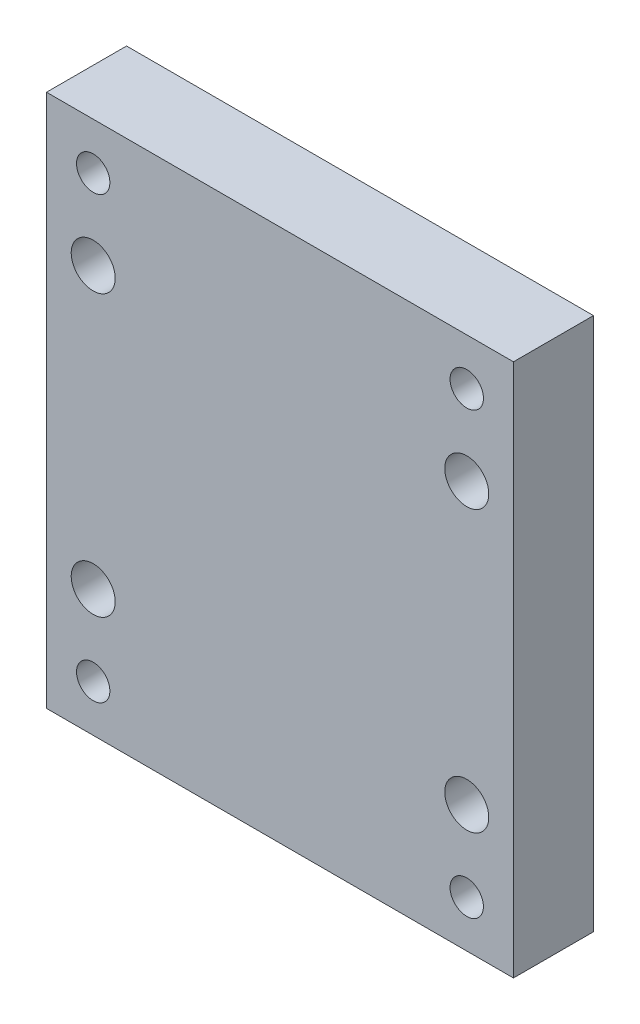
from build123d import *

# Parameters (mm, degrees)
SKETCH_1_W                     = 70
SKETCH_1_H                     = 80
EXTRUDE_1_DEPTH                = 12
HOLE_WIZARD_M6_1_D             = 5
HOLE_WIZARD_M6_1_2_D           = 6.6
HOLE_WIZARD_M6_1_2_CBORE_D     = 11
HOLE_WIZARD_M6_1_2_CBORE_DEPTH = 6.4
CUT_EXTRUDE_1_DEPTH            = 2.5
PATTERN_LINEAR_1_COUNT         = 8
PATTERN_LINEAR_1_PITCH         = 10


with BuildPart() as part:
    # 草图1 → 凸台-拉伸1 (new body)
    with BuildSketch(Plane.XY):
        Rectangle(SKETCH_1_W, SKETCH_1_H)
    extrude(amount=EXTRUDE_1_DEPTH)

    # Hole Wizard M6 _1 (through all)
    with Locations(Plane(origin=(0, 0, 0), x_dir=(-1, 0, 0), z_dir=(0, 0, -1))):
        with Locations((-28, -33), (-28, 33), (28, 33), (28, -33)):
            Hole(HOLE_WIZARD_M6_1_D / 2)

    # Hole Wizard M6 _1 2 (through all)
    with Locations(Plane(origin=(0, 0, 0), x_dir=(-1, 0, 0), z_dir=(0, 0, -1))):
        with Locations((-28, -21), (-28, 21), (28, -21), (28, 21)):
            CounterBoreHole(HOLE_WIZARD_M6_1_2_D / 2, HOLE_WIZARD_M6_1_2_CBORE_D / 2, HOLE_WIZARD_M6_1_2_CBORE_DEPTH)

    # 草图6 → 切除-拉伸1 (cut)
    with BuildSketch(Plane(origin=(0, 0, 0), x_dir=(-1, 0, 0), z_dir=(0, 0, -1))):
        with BuildLine():
            Line((17.5, 32.5), (-17.5, 32.5))
            ThreePointArc((-17.5, 32.5), (-20, 35), (-17.5, 37.5))
            Line((-17.5, 37.5), (17.5, 37.5))
            ThreePointArc((17.5, 37.5), (20, 35), (17.5, 32.5))
        make_face()
    cut_extrude_1 = extrude(amount=-CUT_EXTRUDE_1_DEPTH, mode=Mode.SUBTRACT)

    # 阵列(线性)1: 切除-拉伸1 ×8
    with Locations(*[(0, -i * PATTERN_LINEAR_1_PITCH, 0) for i in range(1, PATTERN_LINEAR_1_COUNT)]):
        add(cut_extrude_1, mode=Mode.SUBTRACT)


solid = part.part
